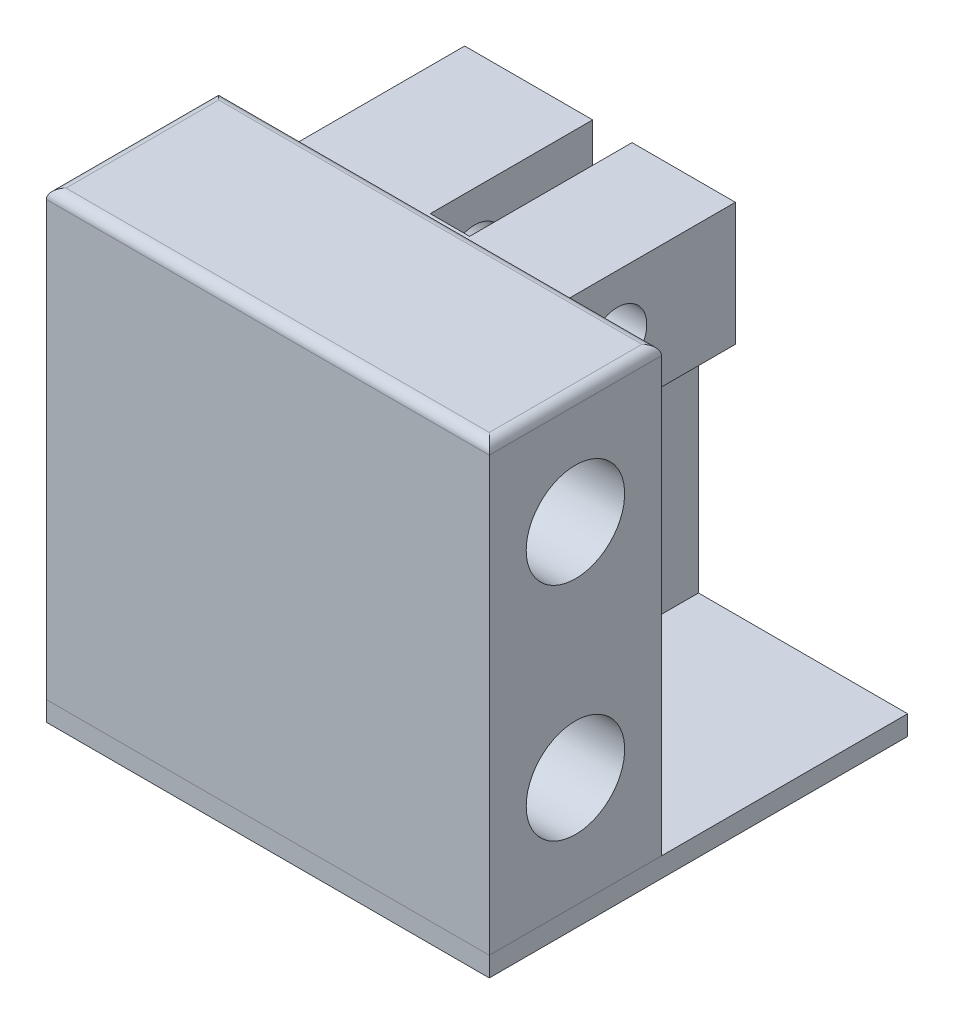
from build123d import *

# Parameters (mm, degrees)
SKETCH1_R           = 10
BOSS_EXTRUDE1_DEPTH = 45
SKETCH1_3_W         = 50
SKETCH1_3_H         = 25
SKETCH1_3_R         = 6
BOSS_EXTRUDE3_DEPTH = 45
BOSS_EXTRUDE4_DEPTH = 45
SKETCH2_R           = 2
SKETCH2_W           = 35
SKETCH2_H           = 50
SKETCH2_W_2         = 8
SKETCH2_H_2         = 33
CUT_EXTRUDE1_DEPTH  = 25
SKETCH3_W           = 50
SKETCH3_H           = 47.5
BOSS_EXTRUDE2_DEPTH = 2.5
FILLET1_R           = 2
SKETCH4_R           = 8
CUT_EXTRUDE2_DEPTH  = 4


with BuildPart() as part:
    # Sketch1 → Boss-Extrude1 (new, symmetric)
    with BuildSketch(Plane(origin=(0, 0, 0), x_dir=(0, 0, -1), z_dir=(1, 0, 0))):
        Polygon((0, 90), (0, 0), (35, 0), (35, 47.5), (35, 72.5), (35, 90), align=None)
        with Locations(Location((17.5, 22.5, 0), (0, 0, 180))):
            Circle(SKETCH1_R, mode=Mode.SUBTRACT)
        with Locations(Location((17.5, 67.5, 0), (0, 0, 180))):
            Circle(SKETCH1_R, mode=Mode.SUBTRACT)
    extrude(amount=BOSS_EXTRUDE1_DEPTH, both=True)

    # Fillet1
    fillet1_edges = [part.edges().sort_by_distance(p)[0] for p in [
        (0, 90, 0),
        (0, 90, -35),
        (45, 90, -17.5),
        (-45, 90, -17.5),
    ]]
    fillet(fillet1_edges, radius=FILLET1_R)


with BuildPart() as body_2:
    # Sketch1<3> → Boss-Extrude3 (new, symmetric)
    with BuildSketch(Plane(origin=(0, 0, 0), x_dir=(0, 0, -1), z_dir=(1, 0, 0))):
        with Locations((60, 60)):
            Rectangle(SKETCH1_3_W, SKETCH1_3_H)
        with Locations(Location((61, 60, 0), (0, 0, 180))):
            Circle(SKETCH1_3_R, mode=Mode.SUBTRACT)
    extrude(amount=BOSS_EXTRUDE3_DEPTH, both=True)

    # Sketch2 → Cut-Extrude1 (cut)
    with BuildSketch(Plane(origin=(0, 72.5, 0), x_dir=(1, 0, 0), z_dir=(0, 1, 0))):
        with Locations(Location((-15, 47, 0), (0, 0, 270))):
            Circle(SKETCH2_R)
        with Locations((27.5, 60)):
            Rectangle(SKETCH2_W, SKETCH2_H)
        with Locations((-15, 68.5)):
            Rectangle(SKETCH2_W_2, SKETCH2_H_2)
    extrude(amount=-CUT_EXTRUDE1_DEPTH, mode=Mode.SUBTRACT)


with BuildPart() as body_3:
    # Sketch1<4> → Boss-Extrude4 (new, symmetric)
    with BuildSketch(Plane(origin=(0, 0, 0), x_dir=(0, 0, -1), z_dir=(1, 0, 0))):
        Polygon((85, 0), (85, -4), (0, -4), (0, 0), (35, 0), align=None)
    extrude(amount=BOSS_EXTRUDE4_DEPTH, both=True)

    # Sketch4 → Cut-Extrude2 (cut)
    with BuildSketch(Plane.XZ.offset(4)):
        with Locations(Location((13.5, -54.5, 0), (0, 0, 270))):
            Circle(SKETCH4_R)
    extrude(amount=-CUT_EXTRUDE2_DEPTH, mode=Mode.SUBTRACT)


with BuildPart() as body_4:
    # Sketch3 → Boss-Extrude2 (new, symmetric)
    with BuildSketch(Plane(origin=(0, 0, 0), x_dir=(0, 0, -1), z_dir=(1, 0, 0))):
        with Locations((60, 23.75)):
            Rectangle(SKETCH3_W, SKETCH3_H)
    extrude(amount=BOSS_EXTRUDE2_DEPTH, both=True)


solid = Compound([part.part, body_2.part, body_3.part, body_4.part])
